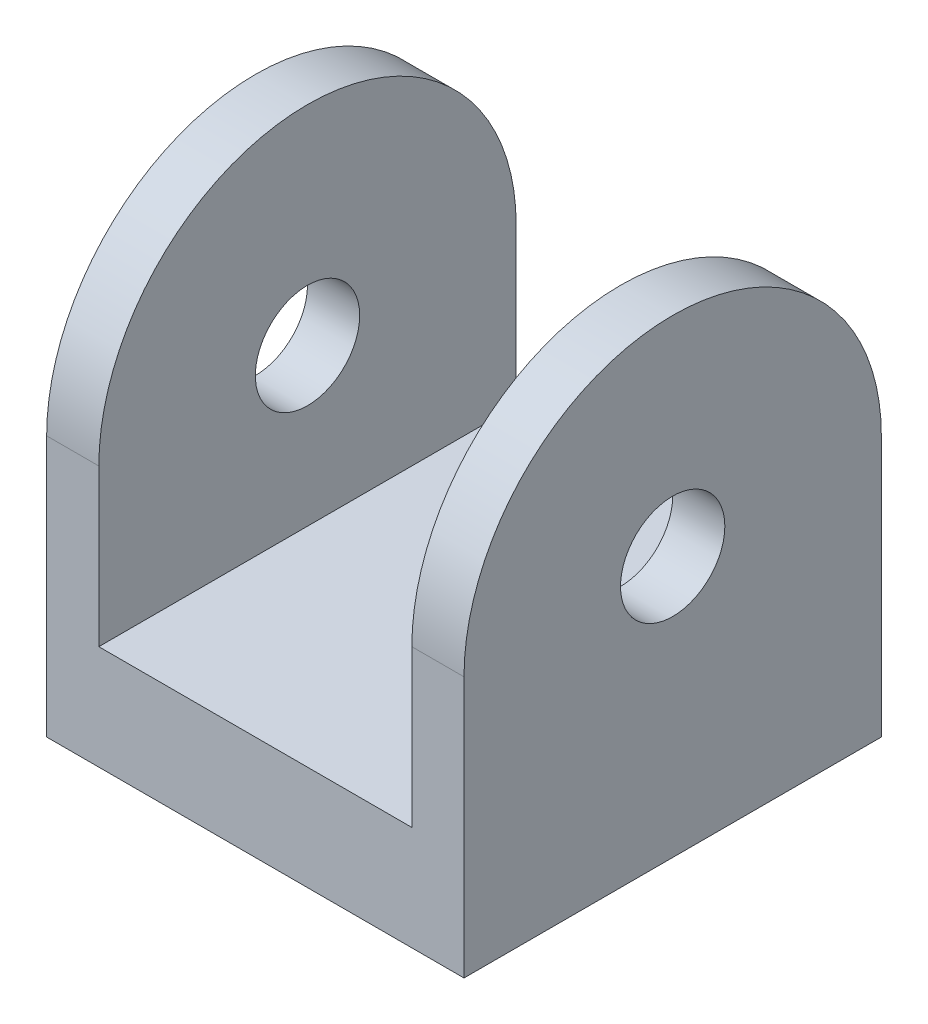
from build123d import *

# Parameters (mm, degrees)
SKETCH1_W           = 40
SKETCH1_H           = 40
BOSS_EXTRUDE1_DEPTH = 10
BOSS_EXTRUDE2_DEPTH = 5
SKETCH4_R           = 5
CUT_EXTRUDE1_DEPTH  = 52.5


with BuildPart() as part:
    # Sketch1 → Boss-Extrude1 (new body)
    with BuildSketch(Plane(origin=(0, 0, 0), x_dir=(1, 0, 0), z_dir=(0, 1, 0))):
        Rectangle(SKETCH1_W, SKETCH1_H)
    extrude(amount=BOSS_EXTRUDE1_DEPTH)

    # Sketch2 → Boss-Extrude2 (add)
    with BuildSketch(Plane(origin=(20, 0, 0), x_dir=(0, 0, -1), z_dir=(1, 0, 0))):
        with BuildLine():
            Line((-20, 10), (-20, 25))
            ThreePointArc((-20, 25), (0, 45), (20, 25))
            Line((20, 25), (20, 10))
            Line((20, 10), (-20, 10))
        make_face()
    boss_extrude2 = extrude(amount=-BOSS_EXTRUDE2_DEPTH)

    # Mirror1: Boss-Extrude2 across plane
    add(boss_extrude2.mirror(Plane(origin=(0, 0, 0), x_dir=(0, 0, 1), z_dir=(1, 0, 0))))

    # Sketch4 → Cut-Extrude1 (cut, symmetric)
    with BuildSketch(Plane(origin=(17.5, 0, 0), x_dir=(0, 0, -1), z_dir=(1, 0, 0))):
        with Locations((0, 25)):
            Circle(SKETCH4_R)
    extrude(amount=CUT_EXTRUDE1_DEPTH, both=True, mode=Mode.SUBTRACT)


solid = part.part
